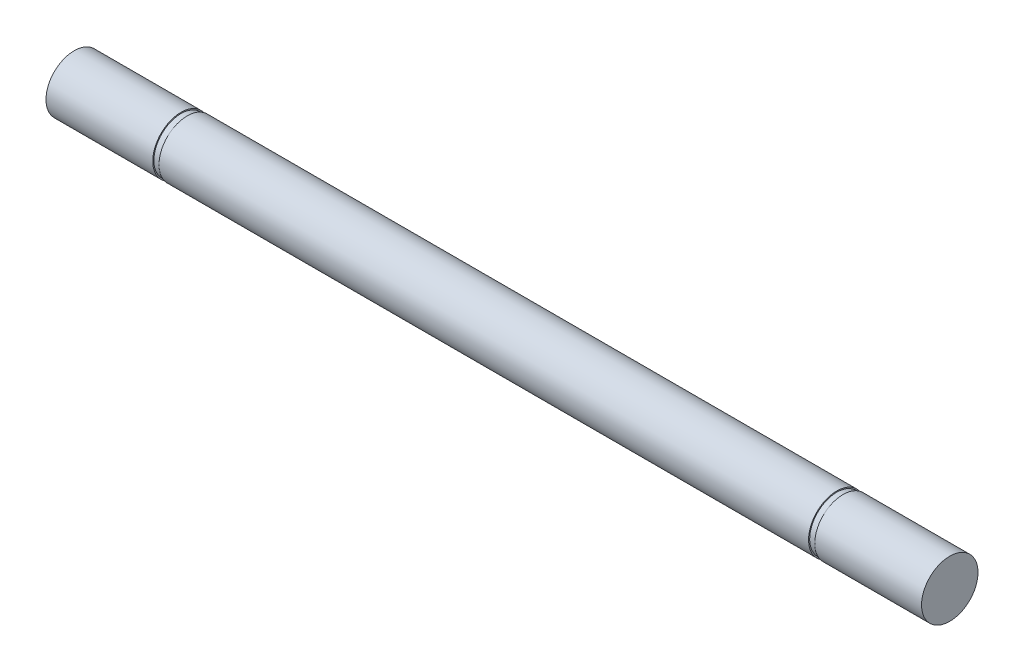
from build123d import *


with BuildPart() as part:
    # Sketch1 → Revolve1 (revolve)
    with BuildSketch(Plane.XY):
        Polygon((-57.596279733, -12.106542056), (-57.596279733, -7.106542056), (-38.696279733, -7.106542056), (-38.696279733, -7.306542056), (-37.596279733, -7.306542056), (-37.596279733, -7.106542056), (77.403720267, -7.106542056), (77.403720267, -7.306542056), (78.503720267, -7.306542056), (78.503720267, -7.106542056), (97.403720267, -7.106542056), (97.403720267, -12.106542056), align=None)
    revolve(axis=Axis((97.403720267, -12.106542056, 0), (-1, 0, 0)))


solid = part.part
